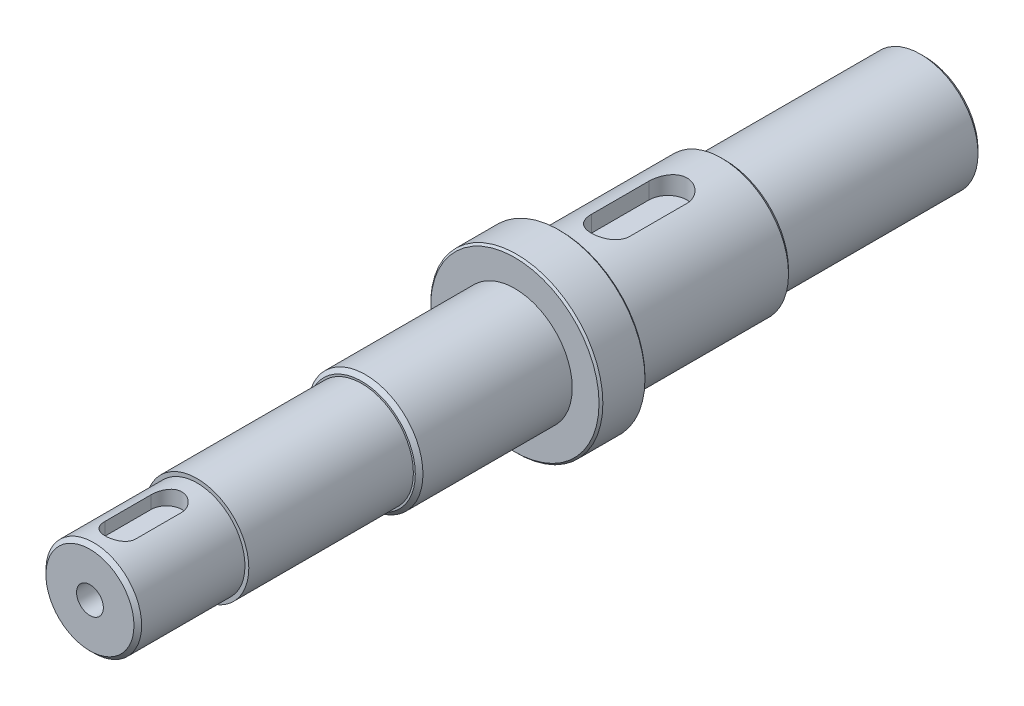
SolidWorks part; units mm, degrees
ref_plane "Front Plane" through (0, 0, 0) normal (0, 0, 1) x (1, 0, 0)
ref_plane "Top Plane" through (0, 0, 0) normal (0, 1, 0) x (1, 0, 0)
ref_plane "Right Plane" through (0, 0, 0) normal (1, 0, 0) x (0, 0, -1)
sketch "Sketch1" plane through (0, 0, 0) normal (0, 0, 1) x (1, 0, 0)
  circle A0 centre (0, 0) radius 15
  dimension "D1" = 30
extrude "Boss-Extrude1" add sketch "Sketch1" along normal blind 52
sketch "Sketch2" plane through (0, 0, 52) normal (0, 0, 1) x (1, 0, 0)
  circle A0 centre (0, 0) radius 17.5
  dimension "D1" = 35
extrude "Boss-Extrude2" add sketch "Sketch2" along normal blind 43
sketch "Sketch3" plane through (0, 0, 95) normal (0, 0, 1) x (1, 0, 0)
  circle A0 centre (0, 0) radius 22.5
extrude "Boss-Extrude3" add sketch "Sketch3" along normal blind 12
sketch "Sketch4" plane through (0, 0, 107) normal (0, 0, 1) x (1, 0, 0)
  circle A0 centre (0, 0) radius 15
  dimension "D1" = 30
extrude "Boss-Extrude4" add sketch "Sketch4" along normal blind 40
sketch "Sketch5" plane through (0, 0, 147) normal (0, 0, 1) x (1, 0, 0)
  circle A0 centre (0, 0) radius 13.5
  dimension "D1" = 27
extrude "Boss-Extrude5" add sketch "Sketch5" along normal blind 43
sketch "Sketch6" plane through (0, 0, 190) normal (0, 0, 1) x (1, 0, 0)
  circle A0 centre (0, 0) radius 12.5
extrude "Boss-Extrude6" add sketch "Sketch6" along normal blind 28
chamfer "Chamfer1" distance 1 angle 45 1 edges at (15, 0, 0)
chamfer "Chamfer2" distance 1 angle 45 3 edges at (12.5, 0, 218) (15, 0, 147) (17.5, 0, 52)
chamfer "Chamfer3" distance 0.5 angle 45 2 edges at (22.5, 0, 107) (22.5, 0, 95)
sketch "Sketch7" plane through (0, 0, 0) normal (0, 1, 0) x (1, 0, 0)
  line L0 (0, -67) -> (0, -82) construction
  line L1 (5, -67) -> (5, -82)
  line L2 (-5, -67) -> (-5, -82)
  line L3 (15, -52) -> (-15, -52) construction
  arc A0 (5, -67) -> (-5, -67) centre (0, -67) ccw
  arc A1 (-5, -82) -> (5, -82) centre (0, -82) ccw
  point P3 (0, -74.5)
  dimension "D1" = 10
  dimension "D2" = 15
  dimension "D3" = 22.5
extrude "Cut-Extrude1" cut sketch "Sketch7" along normal blind 20 from offset 12.5
sketch "Sketch8" plane through (0, 0, 0) normal (0, 1, 0) x (1, 0, 0)
  line L0 (0, -198) -> (0, -210) construction
  line L1 (4, -198) -> (4, -210)
  line L2 (-4, -198) -> (-4, -210)
  line L3 (-11.5, -218) -> (11.5, -218) construction
  arc A0 (4, -198) -> (-4, -198) centre (0, -198) ccw
  arc A1 (-4, -210) -> (4, -210) centre (0, -210) ccw
  point P3 (0, -204)
  dimension "D1" = 14
  dimension "D2" = 8
  dimension "D3" = 12
extrude "Cut-Extrude2" cut sketch "Sketch8" along normal blind 10 from offset 8.5
hole_wizard "M8x1.0 Tapped Hole1" positions "3DSketch1" profile "Sketch9" tap size "M8x1.0" standard "GB"
sketch3d "3DSketch1"
  line L0 (0, 0, 217) -> (0, 0, 218) construction
  point P0 (0, 0, 218)
sketch "Sketch9" plane through (0, 0, 218) normal (1, 0, 0) x (0, -1, 0)
  line L0 (0, 0) -> (0, 21.103)
  line L1 (0, 21.103) -> (3.5, 19)
  line L2 (3.5, 19) -> (3.5, 0)
  line L5 (3.5, 0) -> (0, 0)
  line L10 (0, 21.103) -> (-3.5, 19) construction
  line L11 (0, -6.35) -> (0, 107.95) construction
  dimension "螺纹孔钻头直径" = 7
  dimension "螺纹孔钻头深度" = 19
  dimension "导头角度" = 118
cosmetic thread "Cosmetic Thread 1" parameters "D1"=16, "D2"=8
